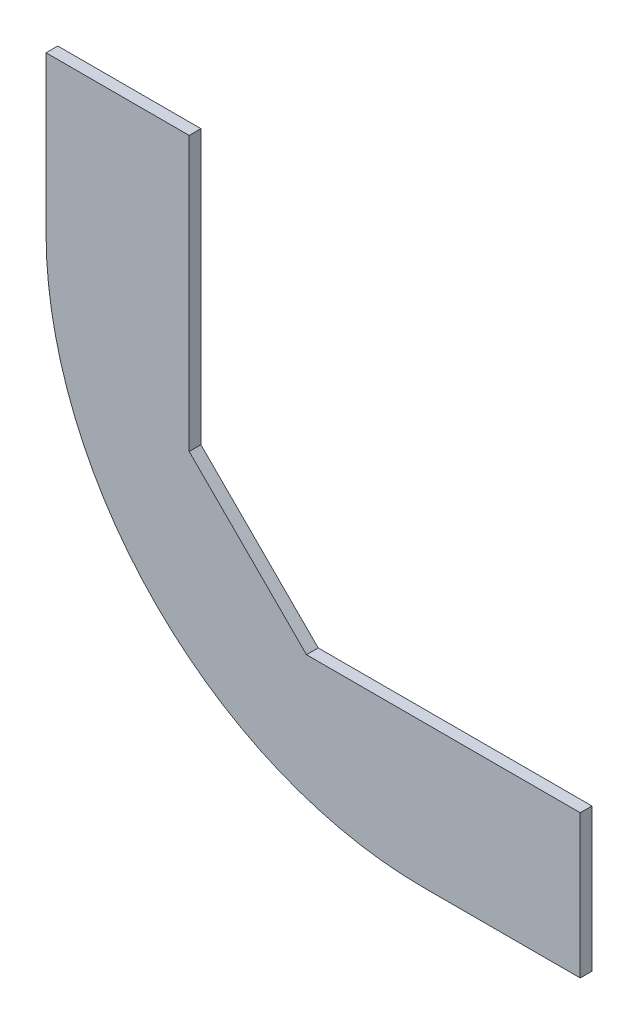
SolidWorks part; units mm, degrees
ref_plane "前视基准面" through (0, 0, 0) normal (0, 0, 1) x (1, 0, 0)
ref_plane "上视基准面" through (0, 0, 0) normal (0, 1, 0) x (1, 0, 0)
ref_plane "右视基准面" through (0, 0, 0) normal (1, 0, 0) x (0, 0, -1)
sketch "草图1" plane through (0, 0, 0) normal (0, 0, 1) x (1, 0, 0)
  line L0 (28.6596, 45.489) -> (28.6596, 25.489)
  line L1 (76.9596, -22.811) -> (96.9596, -22.811)
  line L2 (46.9596, 45.489) -> (46.9596, 10.489)
  line L3 (61.9596, -4.511) -> (96.9596, -4.511)
  line L4 (46.9596, 45.489) -> (46.9596, 25.489) construction
  line L5 (76.9596, -4.511) -> (96.9596, -4.511) construction
  line L6 (46.9596, 10.489) -> (61.9596, -4.511)
  line L7 (28.6596, 45.489) -> (46.9596, 45.489)
  line L8 (96.9596, -4.511) -> (96.9596, -22.811)
  arc A0 (76.9596, -22.811) -> (28.6596, 25.489) centre (76.9596, 25.489) cw
  arc A2 (76.9596, -4.511) -> (46.9596, 25.489) centre (76.9596, 25.489) cw construction
  point P5 (28.6596, -22.811)
  point P13 (46.9596, -4.511)
  dimension "D3" = 48.3
  dimension "D1" = 68.3
  dimension "D2" = 68.3
  dimension "D4" = 18.3
extrude "凸台-拉伸1" add sketch "草图1" along normal blind 1.5
